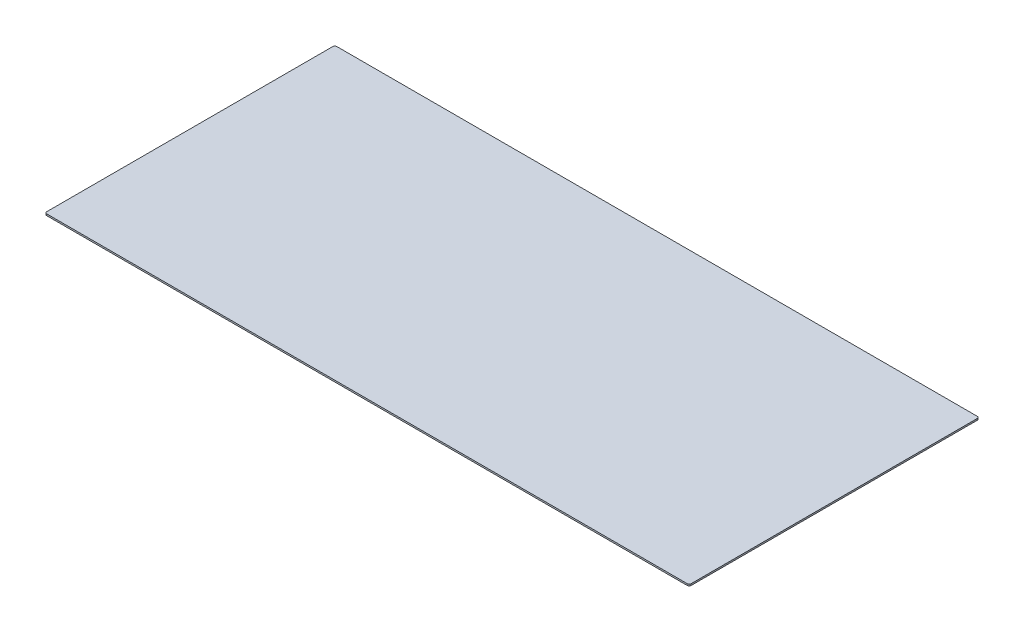
from build123d import *

# Parameters (mm, degrees)
SKETCH1_W           = 2000
SKETCH1_H           = 900
BOSS_EXTRUDE1_DEPTH = 5
FILLET1_R           = 6


with BuildPart() as part:
    # Sketch1 → Boss-Extrude1 (new body)
    with BuildSketch(Plane(origin=(0, 0, 0), x_dir=(1, 0, 0), z_dir=(0, 1, 0))):
        Rectangle(SKETCH1_W, SKETCH1_H)
    extrude(amount=BOSS_EXTRUDE1_DEPTH)

    # Fillet1
    fillet1_edges = [part.edges().sort_by_distance(p)[0] for p in [
        (1000, 2.5, 450),
        (-1000, 2.5, 450),
        (-1000, 2.5, -450),
        (1000, 2.5, -450),
    ]]
    fillet(fillet1_edges, radius=FILLET1_R)


solid = part.part
